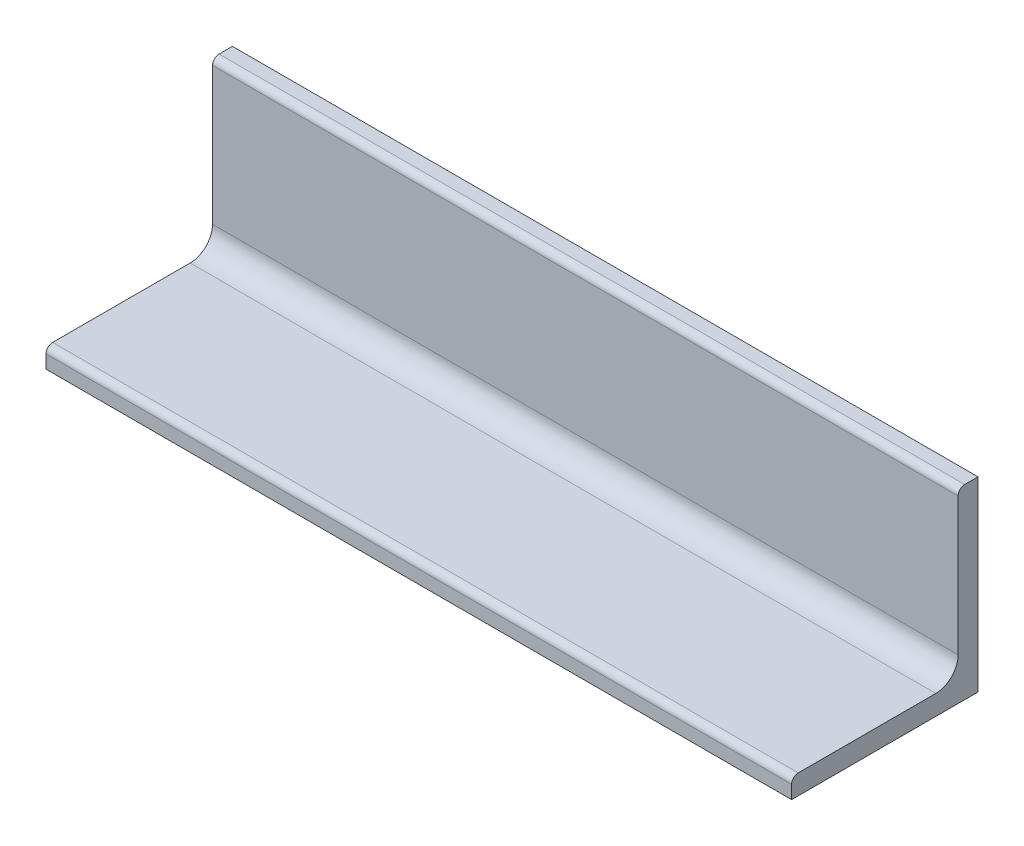
from build123d import *

# Parameters (mm, degrees)
BASE_DEPTH = 300


with BuildPart() as part:
    # Sketch1 → Base (new body)
    with BuildSketch(Plane.YZ):
        with BuildLine():
            Line((0, 75), (0, 0))
            Line((0, 0), (75, 0))
            Line((75, 0), (75, 5.333333333))
            ThreePointArc((75, 5.333333333), (74.218951416, 7.218951416), (72.333333333, 8))
            Line((72.333333333, 8), (17, 8))
            ThreePointArc((17, 8), (10.636038969, 10.636038969), (8, 17))
            Line((8, 17), (8, 72.333333333))
            ThreePointArc((8, 72.333333333), (7.218951416, 74.218951416), (5.333333333, 75))
            Line((5.333333333, 75), (0, 75))
        make_face()
    extrude(amount=BASE_DEPTH)


solid = part.part
